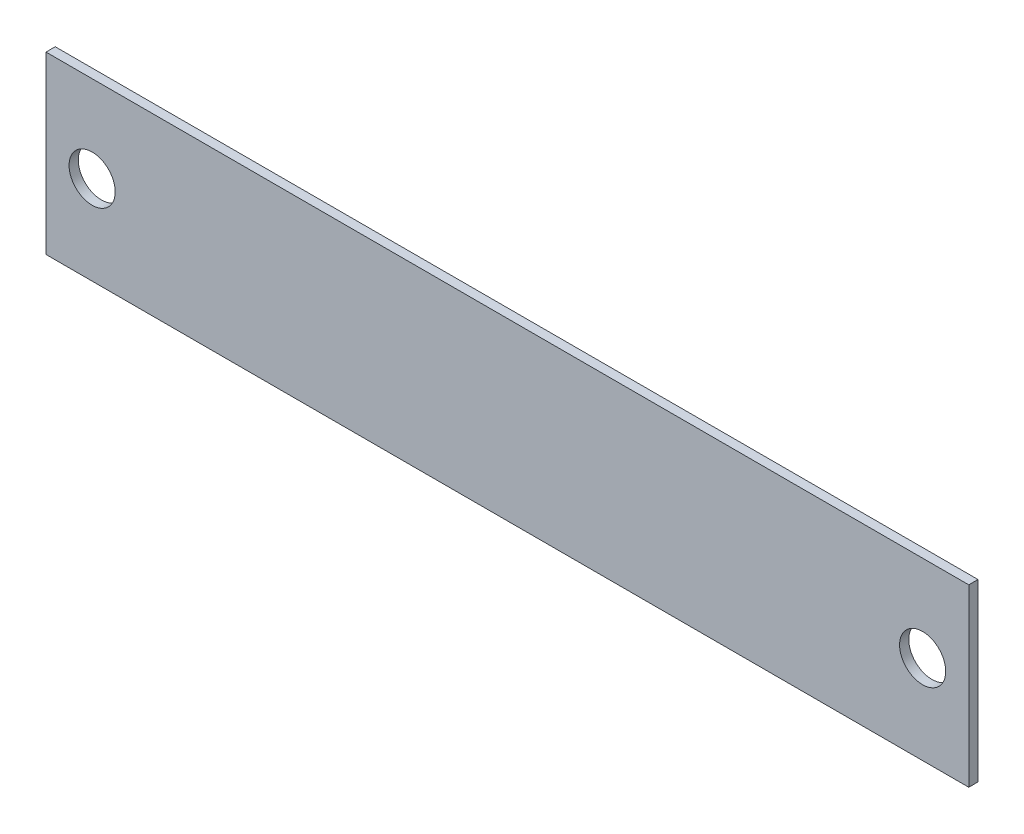
from build123d import *

# Parameters (mm, degrees)
SKETCH_1_W            = 100
SKETCH_1_H            = 19
EXTRUDE_1_DEPTH       = 1
HOLE_WIZARD_5_0_5_1_D = 5


with BuildPart() as part:
    # 草图1 → 凸台-拉伸1 (new body)
    with BuildSketch(Plane.XY):
        with Locations((0, 9.5)):
            Rectangle(SKETCH_1_W, SKETCH_1_H)
    extrude(amount=EXTRUDE_1_DEPTH)

    # Ø5.0 (5) 直径孔1 (through all)
    with Locations(Plane.XY.offset(1)):
        with Locations((-45, 9.621851999), (45, 9.621851999)):
            Hole(HOLE_WIZARD_5_0_5_1_D / 2)


solid = part.part
